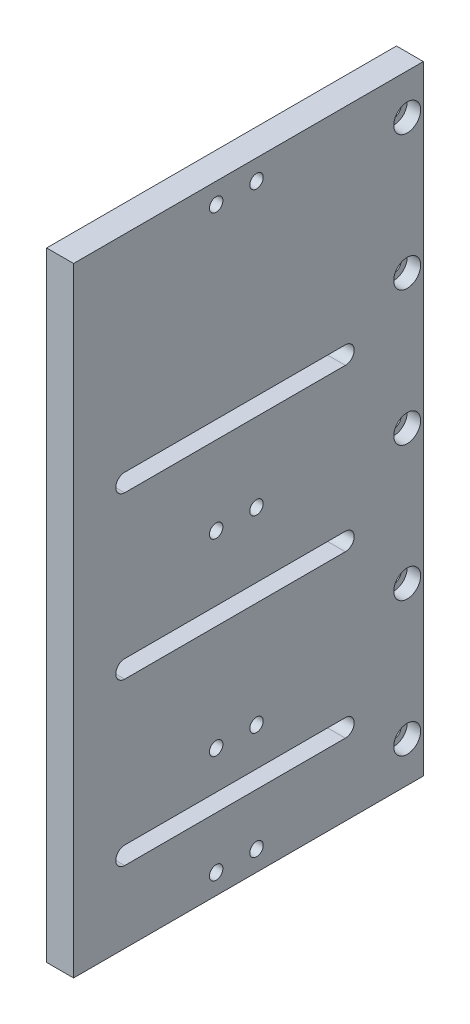
from build123d import *

# Parameters (mm, degrees)
SKETCH_1_W                                         = 130
SKETCH_1_H                                         = 230
BOSS_EXTRUDE_1_DEPTH                               = 10
M6_TAPPED_HOLE_1_D                                 = 5
LINEAR_PATTERN_1_COUNT                             = 2
LINEAR_PATTERN_1_PITCH                             = 15
M5_SOCKET_HEAD_CAP_SCREW_COUNTERBORE_1_D           = 5.5
M5_SOCKET_HEAD_CAP_SCREW_COUNTERBORE_1_CBORE_D     = 10
M5_SOCKET_HEAD_CAP_SCREW_COUNTERBORE_1_CBORE_DEPTH = 5
LINEAR_PATTERN_2_COUNT                             = 3
LINEAR_PATTERN_2_PITCH                             = 50
LINEAR_PATTERN_2_COL_COUNT                         = 3
LINEAR_PATTERN_2_COL_PITCH                         = 50
LINEAR_PATTERN_3_COUNT                             = 2
LINEAR_PATTERN_3_PITCH                             = 110
LINEAR_PATTERN_3_COPY_1_D                          = 5
LINEAR_PATTERN_4_COUNT                             = 2
LINEAR_PATTERN_4_PITCH                             = 215
LINEAR_PATTERN_4_COPY_1_D                          = 5
CUT_EXTRUDE_1_DEPTH                                = 133.476412995
LINEAR_PATTERN_8_COUNT                             = 3
LINEAR_PATTERN_8_PITCH                             = 60
LINEAR_PATTERN_7_COUNT                             = 2
LINEAR_PATTERN_7_PITCH                             = 40
LINEAR_PATTERN_7_COPY_1_D                          = 5


with BuildPart() as part:
    # Sketch 1 → Boss-Extrude 1 (new body)
    with BuildSketch(Plane(origin=(0, 0, 0), x_dir=(0, 0, -1), z_dir=(1, 0, 0))):
        Rectangle(SKETCH_1_W, SKETCH_1_H)
    extrude(amount=BOSS_EXTRUDE_1_DEPTH)

    # M6 Tapped Hole 1 (through all)
    with Locations(Plane.ZY):
        with Locations((12, -107.5)):
            m6_tapped_hole_1 = Hole(M6_TAPPED_HOLE_1_D / 2)

    # Linear Pattern 1: M6 Tapped Hole 1 ×2
    with Locations(*[(0, 0, -i * LINEAR_PATTERN_1_PITCH) for i in range(1, LINEAR_PATTERN_1_COUNT)]):
        add(m6_tapped_hole_1, mode=Mode.SUBTRACT)

    # M5 Socket Head Cap Screw Counterbore 1 (through all)
    with Locations(Plane(origin=(10, 0, 0), x_dir=(0, 0, -1), z_dir=(1, 0, 0))):
        with Locations((59, 0)):
            m5_socket_head_cap_screw_counterbore_1 = CounterBoreHole(M5_SOCKET_HEAD_CAP_SCREW_COUNTERBORE_1_D / 2, M5_SOCKET_HEAD_CAP_SCREW_COUNTERBORE_1_CBORE_D / 2, M5_SOCKET_HEAD_CAP_SCREW_COUNTERBORE_1_CBORE_DEPTH)

    # Linear Pattern 2: M5 Socket Head Cap Screw Counterbore 1 ×3
    with Locations(*[(0, i * LINEAR_PATTERN_2_PITCH, 0) for i in range(1, LINEAR_PATTERN_2_COUNT)]):
        add(m5_socket_head_cap_screw_counterbore_1, mode=Mode.SUBTRACT)

    # Linear Pattern 2 col: M5 Socket Head Cap Screw Counterbore 1 ×3
    with Locations(*[(0, -i * LINEAR_PATTERN_2_COL_PITCH, 0) for i in range(1, LINEAR_PATTERN_2_COL_COUNT)]):
        add(m5_socket_head_cap_screw_counterbore_1, mode=Mode.SUBTRACT)

    # Linear Pattern 3: M6 Tapped Hole 1 ×2
    with Locations(*[(0, i * LINEAR_PATTERN_3_PITCH, 0) for i in range(1, LINEAR_PATTERN_3_COUNT)]):
        add(m6_tapped_hole_1, mode=Mode.SUBTRACT)

    # Linear Pattern 3 copy 1 (through all)
    with Locations(Plane(origin=(0, 110, -15), x_dir=(0, 0, 1), z_dir=(-1, 0, 0))):
        with Locations((12, -107.5)):
            Hole(LINEAR_PATTERN_3_COPY_1_D / 2)

    # Linear Pattern 4: M6 Tapped Hole 1 ×2
    with Locations(*[(0, i * LINEAR_PATTERN_4_PITCH, 0) for i in range(1, LINEAR_PATTERN_4_COUNT)]):
        add(m6_tapped_hole_1, mode=Mode.SUBTRACT)

    # Linear Pattern 4 copy 1 (through all)
    with Locations(Plane(origin=(0, 215, -15), x_dir=(0, 0, 1), z_dir=(-1, 0, 0))):
        with Locations((12, -107.5)):
            Hole(LINEAR_PATTERN_4_COPY_1_D / 2)

    # Sketch 8 → Cut-Extrude 1 (cut, through all)
    with BuildSketch(Plane.ZY):
        with BuildLine():
            Line((-36, -81.7), (46, -81.7))
            ThreePointArc((46, -81.7), (49.3, -85), (46, -88.3))
            Line((46, -88.3), (-36, -88.3))
            ThreePointArc((-36, -88.3), (-39.3, -85), (-36, -81.7))
        make_face()
    cut_extrude_1 = extrude(amount=-CUT_EXTRUDE_1_DEPTH, mode=Mode.SUBTRACT)

    # Linear Pattern 8: Cut-Extrude 1 ×3
    with Locations(*[(0, i * LINEAR_PATTERN_8_PITCH, 0) for i in range(1, LINEAR_PATTERN_8_COUNT)]):
        add(cut_extrude_1, mode=Mode.SUBTRACT)

    # Linear Pattern 7: M6 Tapped Hole 1 ×2
    with Locations(*[(0, i * LINEAR_PATTERN_7_PITCH, 0) for i in range(1, LINEAR_PATTERN_7_COUNT)]):
        add(m6_tapped_hole_1, mode=Mode.SUBTRACT)

    # Linear Pattern 7 copy 1 (through all)
    with Locations(Plane(origin=(0, 40, -15), x_dir=(0, 0, 1), z_dir=(-1, 0, 0))):
        with Locations((12, -107.5)):
            Hole(LINEAR_PATTERN_7_COPY_1_D / 2)


solid = part.part
